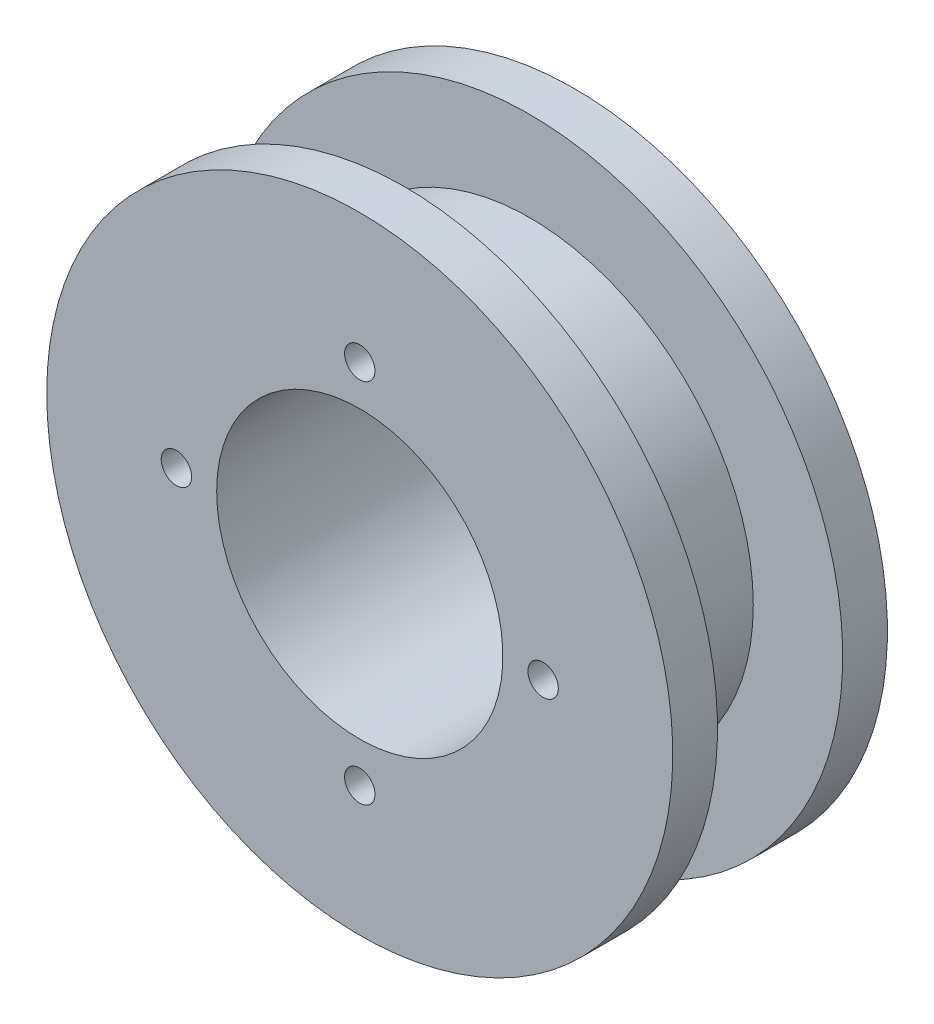
SolidWorks part; units mm, degrees
ref_plane "前视基准面" through (0, 0, 0) normal (0, 0, 1) x (1, 0, 0)
ref_plane "上视基准面" through (0, 0, 0) normal (0, 1, 0) x (1, 0, 0)
ref_plane "右视基准面" through (0, 0, 0) normal (1, 0, 0) x (0, 0, -1)
sketch "草图1" plane through (0, 0, 0) normal (0, 1, 0) x (1, 0, 0)
  line L0 (0, 0) -> (0, -59426.1097) construction
  line L1 (-32, 48) -> (-70, 48)
  line L2 (-70, 48) -> (-70, 38)
  line L3 (-70, 38) -> (-50, 38)
  line L4 (-50, 38) -> (-50, 10)
  line L5 (-50, 10) -> (-70, 10)
  line L6 (-70, 10) -> (-70, 0)
  line L7 (-70, 0) -> (-32, 0)
  line L8 (-32, 48) -> (-32, 0)
  dimension "D1" = 48
  dimension "D2" = 20
  dimension "D3" = 140
  dimension "D4" = 10
  dimension "D5" = 10
  dimension "D6" = 64
revolve "旋转1" add sketch "草图1" angle 360 about L0
hole_wizard "M8 螺纹孔1" positions "草图2" profile "草图3" tap size "M8" standard "GB"
sketch "草图2" plane through (0, 0, -48) normal (0, 0, -1) x (-1, 0, 0)
  circle A0 centre (0, 0) radius 70 construction
  point P0 (0, 41)
  point P2 (41, 0)
  point P4 (-41, 0)
  point P6 (0, -41)
  dimension "D1" = 41
  dimension "D2" = 41
  dimension "D3" = 41
  dimension "D4" = 41
sketch "草图3" plane through (0, 41, -48) normal (1, 0, 0) x (0, 1, 0)
  line L0 (0, 0) -> (0, 21.7929)
  line L1 (0, 21.7929) -> (3.4, 19.75)
  line L2 (3.4, 19.75) -> (3.4, 0)
  line L5 (3.4, 0) -> (0, 0)
  line L10 (0, 21.7929) -> (-3.4, 19.75) construction
  line L11 (0, -6.35) -> (0, 107.95) construction
  dimension "螺纹孔钻头直径" = 6.8
  dimension "螺纹孔钻头深度" = 19.75
  dimension "导头角度" = 118
cosmetic thread "孔螺蚊线1"
cosmetic thread "孔螺蚊线2"
cosmetic thread "孔螺蚊线3"
cosmetic thread "孔螺蚊线4"
hole_wizard "M8 螺纹孔3" positions "草图6" profile "草图7" tap size "M8" standard "GB"
sketch "草图6" plane through (0, 0, 0) normal (0, 0, 1) x (1, 0, 0)
  point P0 (41, 0)
  point P3 (0, -41)
  point P6 (-41, 0)
  point P9 (0, 41)
sketch "草图7" plane through (41, 0, 0) normal (1, 0, 0) x (0, -1, 0)
  line L0 (0, 0) -> (0, 21.7929)
  line L1 (0, 21.7929) -> (3.4, 19.75)
  line L2 (3.4, 19.75) -> (3.4, 0)
  line L5 (3.4, 0) -> (0, 0)
  line L10 (0, 21.7929) -> (-3.4, 19.75) construction
  line L11 (0, -6.35) -> (0, 107.95) construction
  dimension "螺纹孔钻头直径" = 6.8
  dimension "螺纹孔钻头深度" = 19.75
  dimension "导头角度" = 118
cosmetic thread "孔螺蚊线6"
cosmetic thread "孔螺蚊线7"
cosmetic thread "孔螺蚊线8"
cosmetic thread "孔螺蚊线9"
